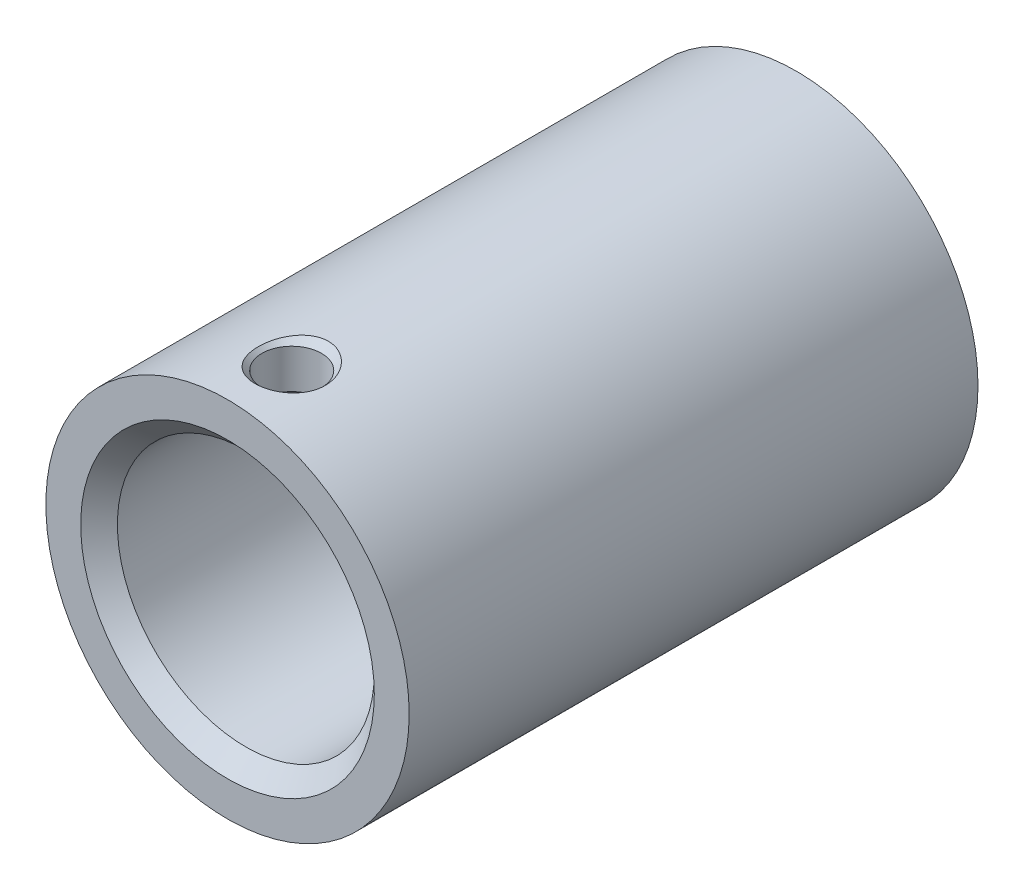
from build123d import *


with BuildPart() as part:
    # 草图1 → 旋转1 (revolve)
    with BuildSketch(Plane(origin=(0, 0, 0), x_dir=(0, 0, -1), z_dir=(1, 0, 0)), mode=Mode.PRIVATE) as revolve_1_sk:
        Polygon((-19, 8), (-18, 7), (12, 7), (12, 9.9), (-19, 9.9), align=None)
    revolve(revolve_1_sk.sketch.rotate(Axis((0, 0, -12), (0, 0, 1)), 270), axis=Axis((0, 0, -12), (0, 0, 1)))

    # 草图2 → 切除-旋转1 (revolve, cut)
    with BuildSketch(Plane(origin=(0, 0, 0), x_dir=(0, 0, -1), z_dir=(1, 0, 0)), mode=Mode.PRIVATE) as cut_revolve_1_sk:
        Polygon((-15.5, 9.9), (-13.5, 9.9), (-13.879, 9.521), (-13.879, 7.379), (-13.5, 7), (-13.5, 0), (-15.5, 0), align=None)
    revolve(cut_revolve_1_sk.sketch.rotate(Axis((0, 0, 15.5), (0, 1, 0)), 180), axis=Axis((0, 0, 15.5), (0, 1, 0)), mode=Mode.SUBTRACT)


solid = part.part
